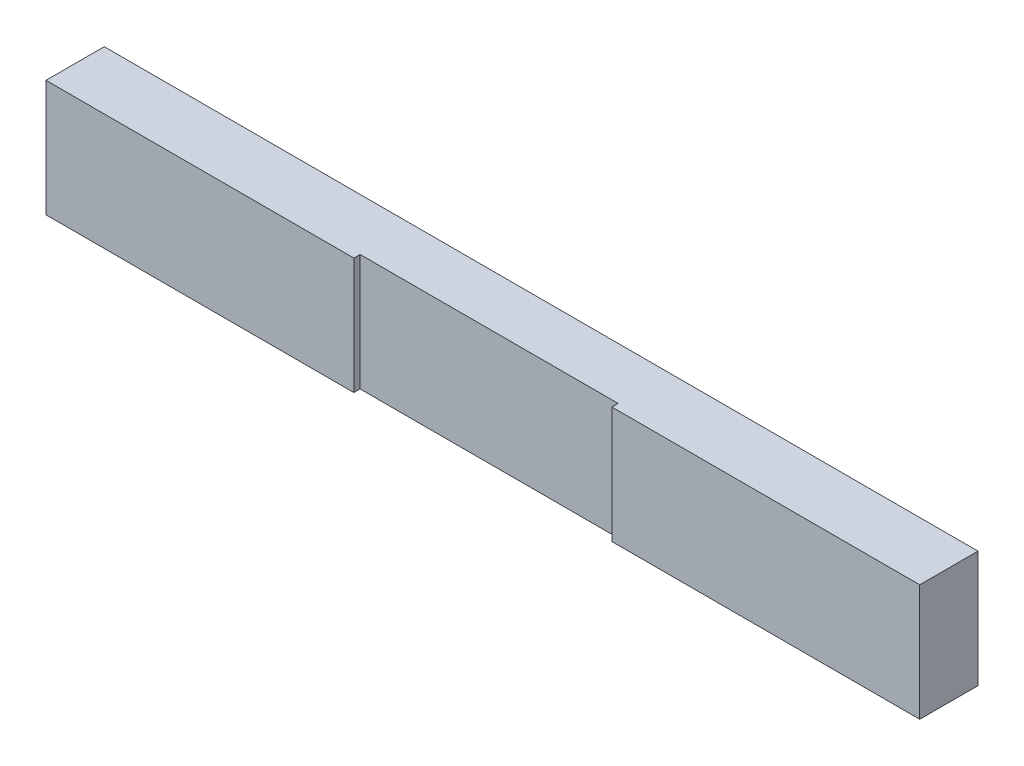
SolidWorks part; units mm, degrees
ref_plane "前视基准面" through (0, 0, 0) normal (0, 0, 1) x (1, 0, 0)
ref_plane "上视基准面" through (0, 0, 0) normal (0, 1, 0) x (1, 0, 0)
ref_plane "右视基准面" through (0, 0, 0) normal (1, 0, 0) x (0, 0, -1)
sketch "草图1" plane through (0, 0, 0) normal (0, 0, 1) x (1, 0, 0)
  line L1 (-105, -14) -> (105, -14)
  line L2 (-105, -14) -> (-105, 14)
  line L3 (-105, 14) -> (105, 14)
  line L4 (105, -14) -> (105, 14)
  line L5 (-105, -14) -> (105, 14) construction
  line L6 (-105, 14) -> (105, -14) construction
  point P0 (0, 0)
  dimension "D1" = 210
  dimension "D2" = 28
extrude "凸台-拉伸1" add sketch "草图1" along normal blind 14
sketch "草图2" plane through (0, 0, 14) normal (0, 0, 1) x (1, 0, 0)
  line L0 (105, 14) -> (-105, 14) construction
  line L1 (-31, -14) -> (31, -14)
  line L2 (-31, -14) -> (-31, 14)
  line L3 (-31, 14) -> (31, 14)
  line L4 (31, -14) -> (31, 14)
  line L5 (-31, -14) -> (31, 14) construction
  line L6 (-31, 14) -> (31, -14) construction
  point P0 (0, 0)
  dimension "D1" = 62
extrude "切除-拉伸1" cut sketch "草图2" against normal blind 1.5
